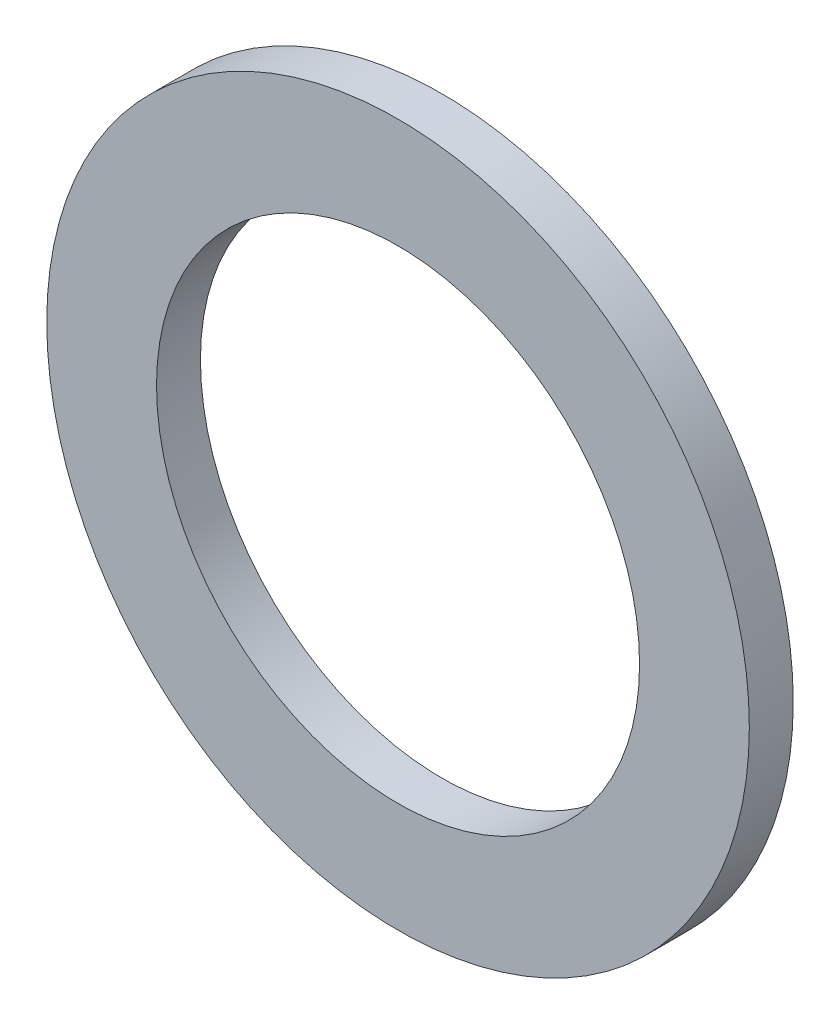
SolidWorks part; units mm, degrees
ref_plane "前视基准面" through (0, 0, 0) normal (0, 0, 1) x (1, 0, 0)
ref_plane "上视基准面" through (0, 0, 0) normal (0, 1, 0) x (1, 0, 0)
ref_plane "右视基准面" through (0, 0, 0) normal (1, 0, 0) x (0, 0, -1)
sketch "草图1" plane through (0, 0, 0) normal (0, 0, 1) x (1, 0, 0)
  circle A0 centre (0, 0) radius 5.5
  circle A1 centre (0, 0) radius 8
  dimension "D1" = 11
  dimension "D2" = 16
extrude "凸台-拉伸1" add sketch "草图1" along normal blind 1
